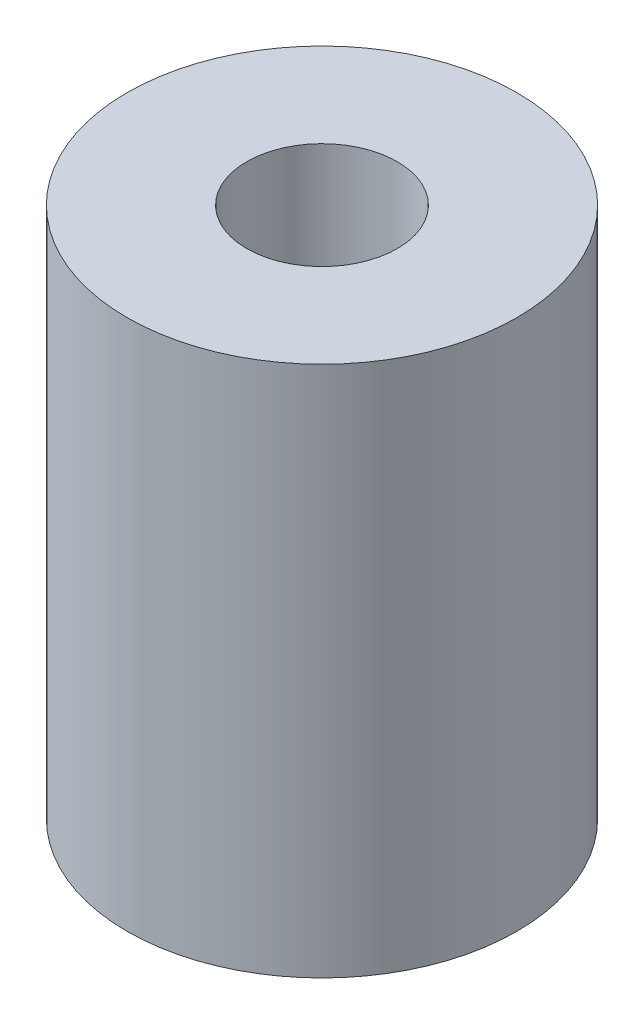
from build123d import *

# Parameters (mm, degrees)
SKETCH1_R              = 11
BOSS_EXTRUDE1_DEPTH    = 30
M10_TAPPED_HOLE1_D     = 8.5
M10_TAPPED_HOLE1_DEPTH = 35
M10_TAPPED_HOLE1_TIP   = 2.553657631


with BuildPart() as part:
    # Sketch1 → Boss-Extrude1 (new body)
    with BuildSketch(Plane(origin=(0, 0, 0), x_dir=(1, 0, 0), z_dir=(0, 1, 0))):
        with Locations(Location((0, 0, 0), (0, 0, 270))):
            Circle(SKETCH1_R)
    extrude(amount=BOSS_EXTRUDE1_DEPTH)

    # M10 Tapped Hole1
    with Locations(Plane(origin=(0, 30, 0), x_dir=(1, 0, 0), z_dir=(0, 1, 0))):
        with Locations((0, 0)):
            Hole(M10_TAPPED_HOLE1_D / 2, depth=M10_TAPPED_HOLE1_DEPTH)
            with Locations((0, 0, -(M10_TAPPED_HOLE1_DEPTH + M10_TAPPED_HOLE1_TIP / 2))):  # 118° drill point
                Cone(0, M10_TAPPED_HOLE1_D / 2, M10_TAPPED_HOLE1_TIP, mode=Mode.SUBTRACT)


solid = part.part
